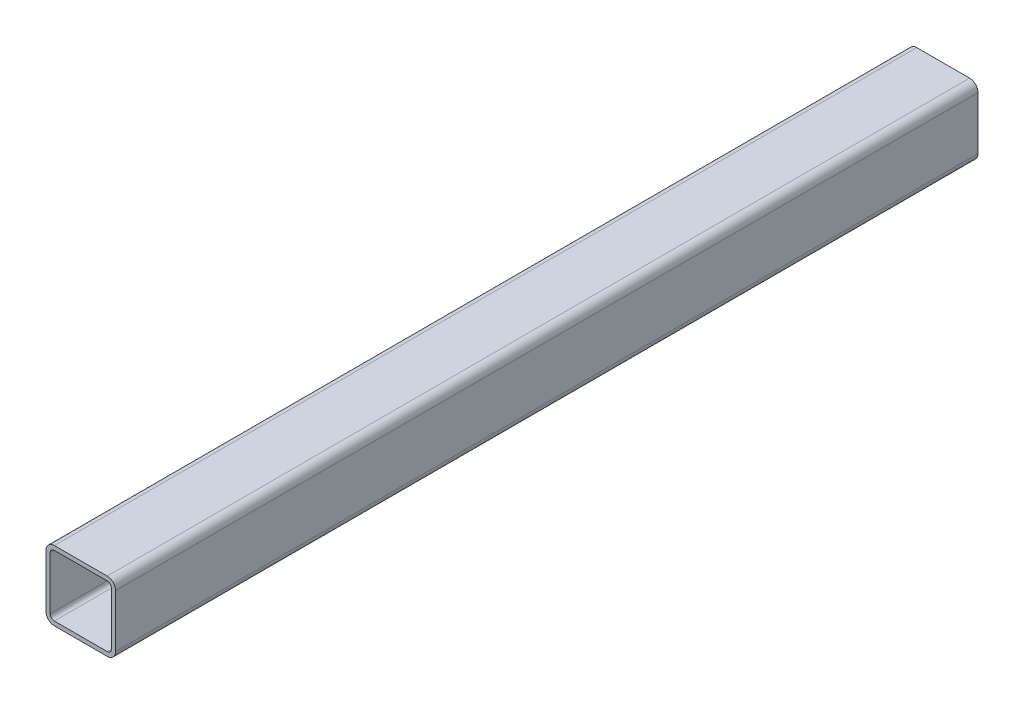
SolidWorks part; units mm, degrees
material "Q235B"
ref_plane "前视基准面" through (0, 0, 0) normal (0, 0, 1) x (1, 0, 0)
ref_plane "上视基准面" through (0, 0, 0) normal (0, 1, 0) x (1, 0, 0)
ref_plane "右视基准面" through (0, 0, 0) normal (1, 0, 0) x (0, 0, -1)
other "Configuration Table"
sketch "草图1" plane through (0, 0, 0) normal (1, 0, 0) x (0, 0, -1)
  line L0 (-310, 0) -> (310, 0)
other "Gb／6728-1986方形空心型钢 050 X 50 X 3(1)"
ref_plane "基准面1" through (0, 0, 310) normal (0, 0, -1) x (0, 1, 0)
sketch "Sketch1" plane through (0, 0, 310) normal (0, 0, -1) x (0, 1, 0)
  line L0 (-19, -22) -> (19, -22)
  line L1 (-22, -19) -> (-22, 19)
  line L2 (19, 22) -> (-19, 22)
  line L3 (22, 19) -> (22, -19)
  line L4 (-19, -25) -> (19, -25)
  line L5 (-25, -19) -> (-25, 19)
  line L6 (19, 25) -> (-19, 25)
  line L7 (25, 19) -> (25, -19)
  arc A0 (25, 19) -> (19, 25) centre (19, 19) ccw
  arc A1 (19, -25) -> (25, -19) centre (19, -19) ccw
  arc A2 (-25, -19) -> (-19, -25) centre (-19, -19) ccw
  arc A3 (-19, 25) -> (-25, 19) centre (-19, 19) ccw
  arc A4 (-19, 22) -> (-22, 19) centre (-19, 19) ccw
  arc A5 (22, 19) -> (19, 22) centre (19, 19) ccw
  arc A6 (19, -22) -> (22, -19) centre (19, -19) ccw
  arc A7 (-22, -19) -> (-19, -22) centre (-19, -19) ccw
  point P0 (-25, 0)
  point P1 (25, 0)
  point P2 (0, 25)
  point P3 (0, -25)
  point P4 (0, 0)
  point P5 (-25, -25)
  point P6 (25, -25)
  point P7 (25, 25)
  point P8 (-25, 25)
  point P33 (0, 0)
  dimension "D1" = 6
  dimension "Thickness" = 3
  dimension "V_leg" = 50
equation "\"D2@草图1\"=\"D1@草图1\"/2"
